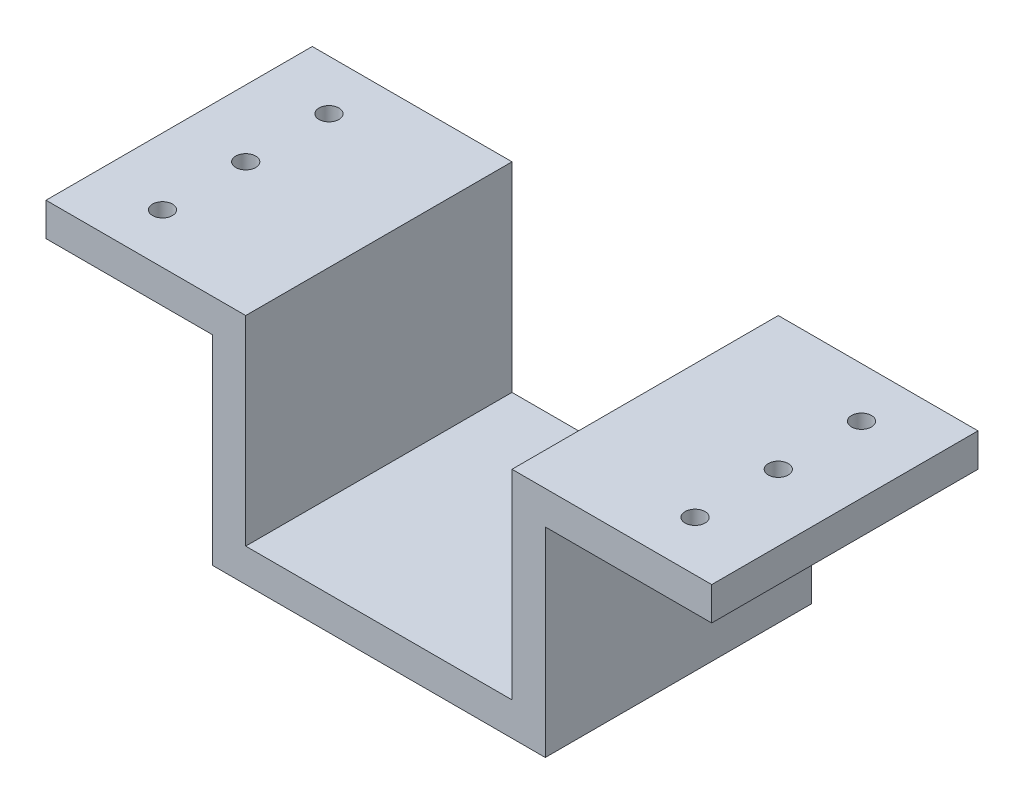
from build123d import *

# Parameters (mm, degrees)
BOSS_EXTRUDE1_DEPTH = 40
SKETCH2_R           = 1.5
CUT_EXTRUDE1_DEPTH  = 73.972597597


with BuildPart() as part:
    # Sketch1 → Boss-Extrude1 (new body)
    with BuildSketch(Plane.XY):
        Polygon((0, 0), (-25, 0), (-25, 30), (-50, 30), (-50, 35), (-20, 35), (-20, 5), (0, 5), (20, 5), (20, 35), (50, 35), (50, 30), (25, 30), (25, 0), align=None)
    extrude(amount=BOSS_EXTRUDE1_DEPTH)

    # Sketch2 → Cut-Extrude1 (cut, through all)
    with BuildSketch(Plane(origin=(0, 35, 0), x_dir=(1, 0, 0), z_dir=(0, 1, 0))):
        with Locations(Location((-40, -7.5, 0), (0, 0, 180))):
            Circle(SKETCH2_R)
        with Locations(Location((-40, -20, 0), (0, 0, 180))):
            Circle(SKETCH2_R)
        with Locations(Location((-40, -32.5, 0), (0, 0, 180))):
            Circle(SKETCH2_R)
        with Locations(Location((40, -7.5, 0), (0, 0, 180))):
            Circle(SKETCH2_R)
        with Locations(Location((40, -20, 0), (0, 0, 180))):
            Circle(SKETCH2_R)
        with Locations(Location((40, -32.5, 0), (0, 0, 180))):
            Circle(SKETCH2_R)
    extrude(amount=-CUT_EXTRUDE1_DEPTH, mode=Mode.SUBTRACT)


solid = part.part
